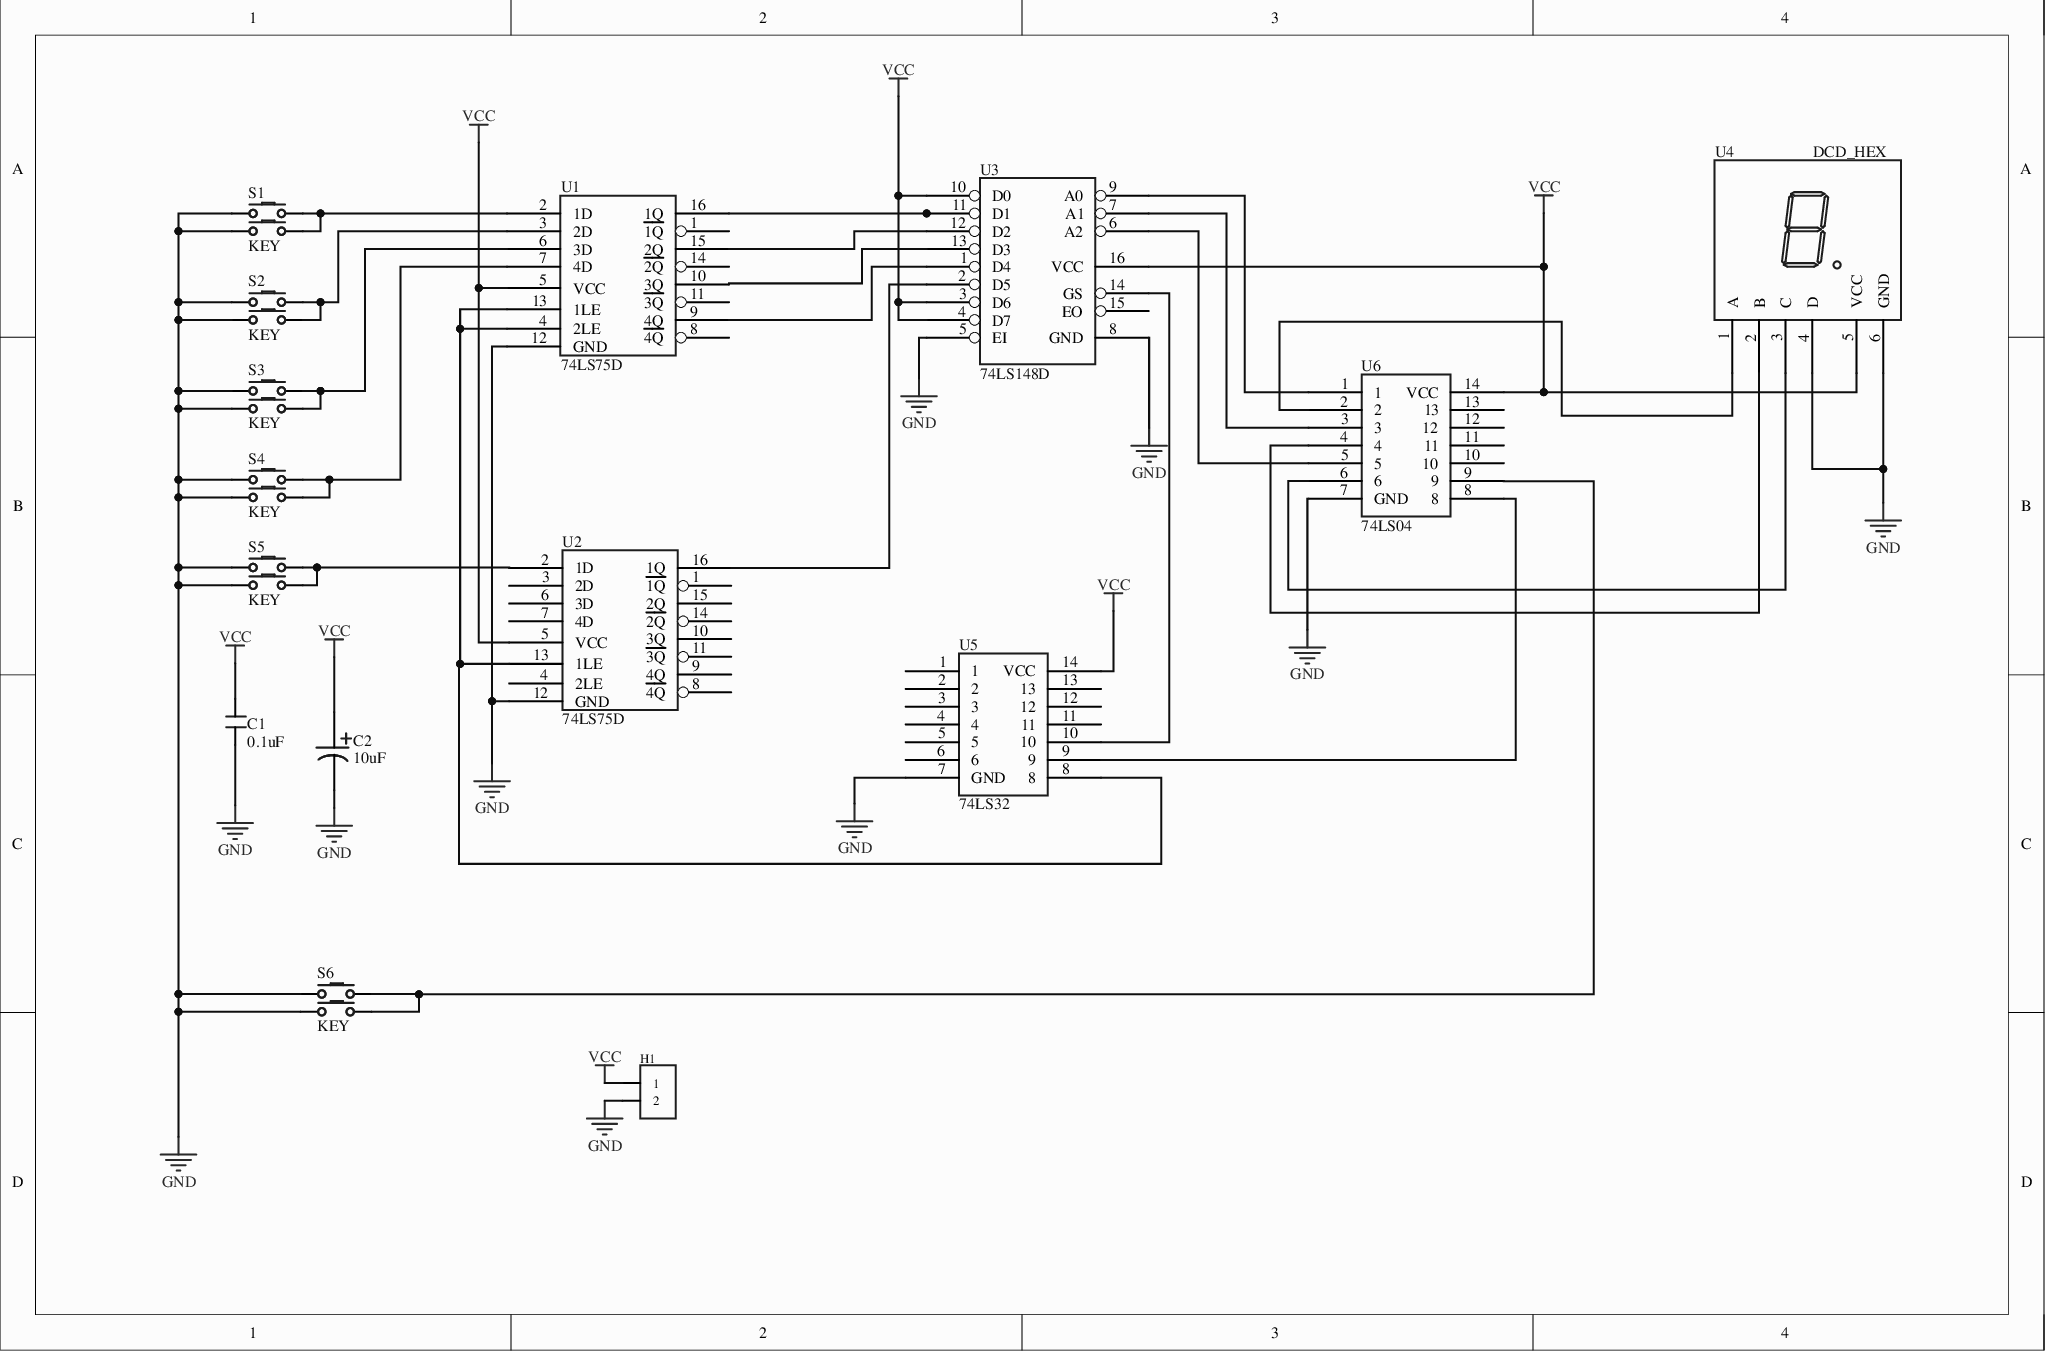
[diagram p0: MISC51507-3.schdoc]
# Altium project MISC51507-2.PrjPcb
1 sheet, 15 parts. Net scope: global (net labels, ports and power ports of the same name join across sheets).
Board file: MISC51507.pcbdoc

## Sheet MISC51507-3.schdoc
size 292 x 193 mm; SheetNumber: 1; SheetTotal: 1; Name: MISC51507

### Parts
C1  0.1uF  [CAP]
C2  10uF  [CAP POL]
H1  (no value)  [HDR-TH_2P-P2.54-V-F]
S1  KEY  [KEY-4]
S2  KEY  [KEY-4]
S3  KEY  [KEY-4]
S4  KEY  [KEY-4]
S5  KEY  [KEY-4]
S6  KEY  [KEY-4]
U1  74LS75D  [74LS75D]
U2  74LS75D  [74LS75D]
U3  74LS148D  [74LS148D]
U4  DCD_HEX  [SMG]
U5  74LS32  [74LS32]
U6  74LS04  [74LS04]

### Nets
GND: C1.1 C2.2 H1.2 S1.1 S1.3 S2.1 S2.3 S3.1 S3.3 S4.1 S4.3 S5.1 S5.3 S6.1 S6.3 U1.12(GND) U2.12(GND) U3.5(EI) U3.8(GND) U4.4(D) U4.6(GND) U5.7(GND) U6.7(GND)
VCC: C1.2 C2.1 H1.1 U1.5(VCC) U2.5(VCC) U3.3(D6) U3.4(D7) U3.10(D0) U3.16(VCC) U4.5(VCC) U5.14(VCC) U6.14(VCC)
NetS1_2: S1.2 S1.4 U1.2(1D)
NetS2_2: S2.2 S2.4 U1.3(2D)
NetS3_2: S3.2 S3.4 U1.6(3D)
NetS4_2: S4.2 S4.4 U1.7(4D)
NetS5_2: S5.2 S5.4 U2.2(1D)
NetS6_2: S6.2 S6.4 U6.9
NetU1_4: U1.4(2LE) U1.13(1LE) U2.13(1LE) U5.8
NetU1_9: U1.9(4Q) U3.1(D4)
NetU1_10: U1.10(3Q) U3.13(D3)
NetU1_15: U1.15(2Q) U3.12(D2)
NetU1_16: U1.16(1Q) U3.11(D1)
NetU2_16: U2.16(1Q) U3.2(D5)
NetU3_6: U3.6(A2) U6.5
NetU3_7: U3.7(A1) U6.3
NetU3_9: U3.9(A0) U6.1
NetU3_14: U3.14(GS) U5.10
NetU4_1: U4.1(A) U6.2
NetU4_2: U4.2(B) U6.4
NetU4_3: U4.3(C) U6.6
NetU5_9: U5.9 U6.8

Not connected (* = marked no-connect by the designer): U1 1(~{1Q})* 8(~{4Q})* 11(~{3Q})* 14(~{2Q})*; U2 1(~{1Q}) 3(2D)* 4(2LE) 6(3D)* 7(4D)* 8(~{4Q}) 9(4Q) 10(3Q) 11(~{3Q}) 14(~{2Q}) 15(2Q); U3 15(EO)*; U5 1 2 3 4 5 6 11 12 13; U6 10 11 12 13

### Library data of the parts
C1 = Cap: UniqueId: b4693cfd16d534cd; AddInBom: yes; Device: Cap; DesignItemID: Cap; LibraryName: PCB; SymbolName: Cap; FootprintName: CAP
C2 = Cap Pol: UniqueId: a2c5d49bc5dde298; AddInBom: yes; Device: Cap Pol; DesignItemID: Cap Pol; LibraryName: PCB; SymbolName: Cap Pol; FootprintName: CAP POL
H1 = HDR-F_2.54_1x2P: Symbol: Header-Female-2.54_1x2; ConvertToPcb: yes; ModelId: a9450ef445564560a104363b9aacde4e0819f05c4eef4c71ace90d822a990e87; ModelName: HDR-TH_2P-P2.54-F-LI-1X2P; ModelTransform: 215.7476,98.425,0,0,0,0,0,0,-129.921; Device: HDR-F_2.54_1x2P; AddInBom: yes; SupplierPart: C49661; Supplier Footprint: 插件; FootprintName: HDR-TH_2P-P2.54-V-F
S1 = KEY-4: UniqueId: 0ac0bd892f9b1ec0; AddInBom: yes; Device: KEY-4; DesignItemID: KEY-4; LibraryName: PCB; SymbolName: KEY-4; FootprintName: KEY-4
S2 = KEY-4: UniqueId: 16ca49f37df57620; AddInBom: yes; Device: KEY-4; DesignItemID: KEY-4; LibraryName: PCB; SymbolName: KEY-4; FootprintName: KEY-4
S3 = KEY-4: UniqueId: b21ed8cc1c3b642b; AddInBom: yes; Device: KEY-4; DesignItemID: KEY-4; LibraryName: PCB; SymbolName: KEY-4; FootprintName: KEY-4
S4 = KEY-4: UniqueId: b4af5bc4dd85243d; AddInBom: yes; Device: KEY-4; DesignItemID: KEY-4; LibraryName: PCB; SymbolName: KEY-4; FootprintName: KEY-4
S5 = KEY-4: UniqueId: b2403b9688924408; AddInBom: yes; Device: KEY-4; DesignItemID: KEY-4; LibraryName: PCB; SymbolName: KEY-4; FootprintName: KEY-4
S6 = KEY-4: UniqueId: 30ed59e7372531b3; AddInBom: yes; Device: KEY-4; DesignItemID: KEY-4; LibraryName: PCB; SymbolName: KEY-4; FootprintName: KEY-4
U1 = 74LS75D: UniqueId: 1bdc0ab44f99f92d; AddInBom: yes; Device: 74LS75D; DesignItemID: 74LS75D; LibraryName: PCB; SymbolName: 74LS75D
U2 = 74LS75D: UniqueId: 48f0ae2437312dae; AddInBom: yes; Device: 74LS75D; DesignItemID: 74LS75D; LibraryName: PCB; SymbolName: 74LS75D
U3 = 74LS148D: UniqueId: 66797bcd97f4f6c2; AddInBom: yes; Device: 74LS148D; DesignItemID: 74LS148D; LibraryName: PCB; SymbolName: 74LS148D; FootprintName: 74LS148D
U4 = SMG: UniqueId: bac468049775df37; AddInBom: yes; Device: SMG; DesignItemID: SMG; LibraryName: five; SymbolName: SMG; FootprintName: SMG
U5 = 74LS32: UniqueId: adf583383e4d69d4; AddInBom: yes; Device: 74LS32; DesignItemID: 74LS32; LibraryName: PCB; SymbolName: 74LS32; FootprintName: 74LS32
U6 = 74LS04: UniqueId: 124c013cfc851acc; AddInBom: yes; Device: 74LS04; DesignItemID: 74LS04; LibraryName: PCB; SymbolName: 74LS04; FootprintName: 74LS04